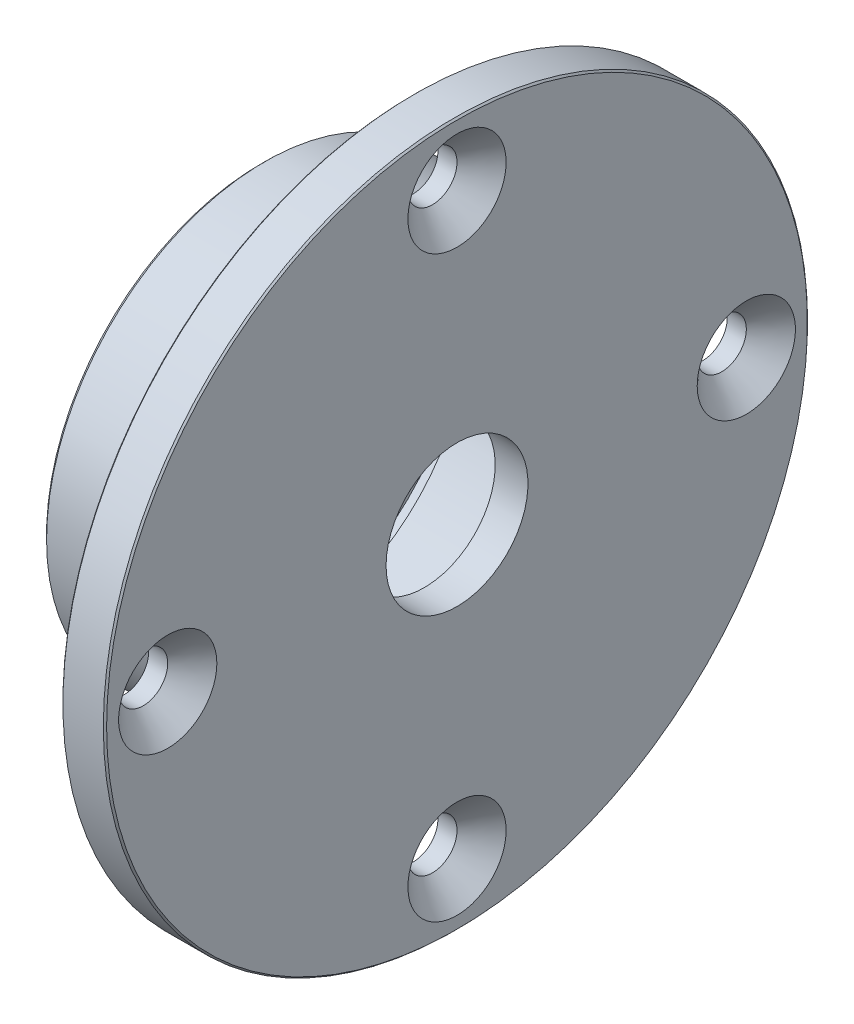
from build123d import *

# Parameters (mm, degrees)
CIRPATTERN1_COUNT  = 4
CHAMFER1_SIZE      = 0.4
SKETCH8_R          = 6.5
CUT_EXTRUDE1_DEPTH = 10
SKETCH9_R          = 33
SKETCH9_R_2        = 32.25
CUT_EXTRUDE2_DEPTH = 10


with BuildPart() as part:
    # Sketch1 → Revolve1 (revolve)
    with BuildSketch(Plane.XY, mode=Mode.PRIVATE) as revolve1_sk:
        Polygon((0, 16), (1.695369244, 16), (1.695369244, 16.85), (2.995369244, 16.85), (2.995369244, 16), (13, 16), (13, 12.5), (15, 12.5), (15, 0), (18, 0), (18, 32.5), (14, 32.5), (14, 20), (0, 20), align=None)
    revolve(revolve1_sk.sketch.rotate(Axis((15, 0, 0), (1, 0, 0)), 90), axis=Axis((15, 0, 0), (1, 0, 0)))

    # Sketch2 → Cut-Revolve1 (revolve, cut)
    with BuildSketch(Plane(origin=(0, 0, 0), x_dir=(1, 0, 0), z_dir=(0, 1, 0)), mode=Mode.PRIVATE) as cut_revolve1_sk:
        Polygon((14, 26.5), (18, 26.5), (18, 31), (15.75, 28.75), (14, 28.75), align=None)
    cut_revolve1 = revolve(cut_revolve1_sk.sketch.rotate(Axis((14, 0, -26.5), (1, 0, 0)), 180), axis=Axis((14, 0, -26.5), (1, 0, 0)), mode=Mode.SUBTRACT)

    # CirPattern1: Cut-Revolve1 ×4 about axis
    cirpattern1_axis = Axis((0, 0, 0), (1, 0, 0))
    for i in range(1, CIRPATTERN1_COUNT):
        add(cut_revolve1.rotate(cirpattern1_axis, i * 360 / CIRPATTERN1_COUNT), mode=Mode.SUBTRACT)

    # Chamfer1
    chamfer1_edges = [part.edges().sort_by_distance(p)[0] for p in [
        (14, 0, -32.5),
        (18, 0, -32.5),
        (13, 0, -12.5),
        (0, 0, -16),
        (0, 0, -20),
    ]]
    chamfer(chamfer1_edges, length=CHAMFER1_SIZE)

    # Sketch8 → Cut-Extrude1 (cut)
    with BuildSketch(Plane.ZY.offset(-15)):
        Circle(SKETCH8_R)
    extrude(amount=-CUT_EXTRUDE1_DEPTH, mode=Mode.SUBTRACT)

    # Sketch9 → Cut-Extrude2 (cut)
    with BuildSketch(Plane(origin=(18, 0, 0), x_dir=(0, 0, -1), z_dir=(1, 0, 0))):
        Circle(SKETCH9_R)
        Circle(SKETCH9_R_2, mode=Mode.SUBTRACT)
    extrude(amount=-CUT_EXTRUDE2_DEPTH, mode=Mode.SUBTRACT)


solid = part.part
